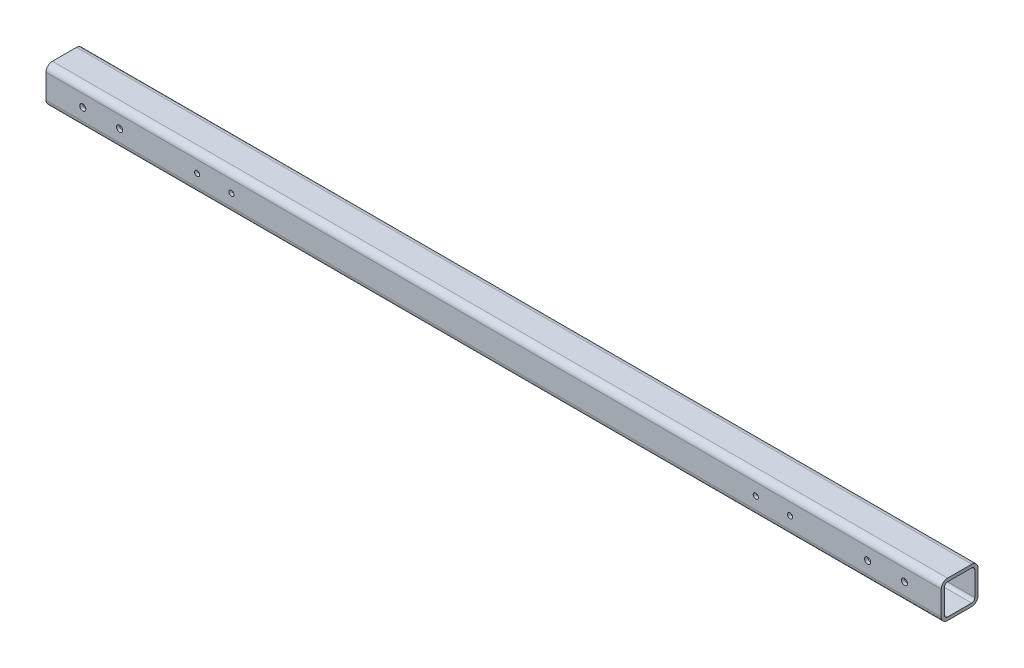
from build123d import *

# Parameters (mm, degrees)
MEMBER_1_DEPTH     = 730
HOLE_WIZARD_M5_1_D = 4.2
HOLE_WIZARD_M6_1_D = 5


with BuildPart() as part:
    # Sketch1 → Member 1 (new body)
    with BuildSketch(Plane(origin=(0, 0, 0), x_dir=(0, 0, -1), z_dir=(1, 0, 0))):
        with BuildLine():
            Line((-9.8, -15), (9.8, -15))
            ThreePointArc((9.8, -15), (13.476955262, -13.476955262), (15, -9.8))
            Line((15, -9.8), (15, 9.8))
            ThreePointArc((15, 9.8), (13.476955262, 13.476955262), (9.8, 15))
            Line((9.8, 15), (-9.8, 15))
            ThreePointArc((-9.8, 15), (-13.476955262, 13.476955262), (-15, 9.8))
            Line((-15, 9.8), (-15, -9.8))
            ThreePointArc((-15, -9.8), (-13.476955262, -13.476955262), (-9.8, -15))
        make_face()
        with BuildLine():
            Line((-9.8, -12.4), (9.8, -12.4))
            ThreePointArc((9.8, -12.4), (11.638477631, -11.638477631), (12.4, -9.8))
            Line((12.4, -9.8), (12.4, 9.8))
            ThreePointArc((12.4, 9.8), (11.638477631, 11.638477631), (9.8, 12.4))
            Line((9.8, 12.4), (-9.8, 12.4))
            ThreePointArc((-9.8, 12.4), (-11.638477631, 11.638477631), (-12.4, 9.8))
            Line((-12.4, 9.8), (-12.4, -9.8))
            ThreePointArc((-12.4, -9.8), (-11.638477631, -11.638477631), (-9.8, -12.4))
        make_face(mode=Mode.SUBTRACT)
    extrude(amount=MEMBER_1_DEPTH)

    # M5 螺纹孔1 (through all)
    with Locations(Plane.XY.offset(15)):
        with Locations((123.2, 0), (151.2, 0), (606.8, 0), (578.8, 0)):
            Hole(HOLE_WIZARD_M5_1_D / 2)

    # M6 螺纹孔1 (through all)
    with Locations(Plane.XY.offset(15)):
        with Locations((30, 0), (60, 0), (700, 0), (670, 0)):
            Hole(HOLE_WIZARD_M6_1_D / 2)


solid = part.part
